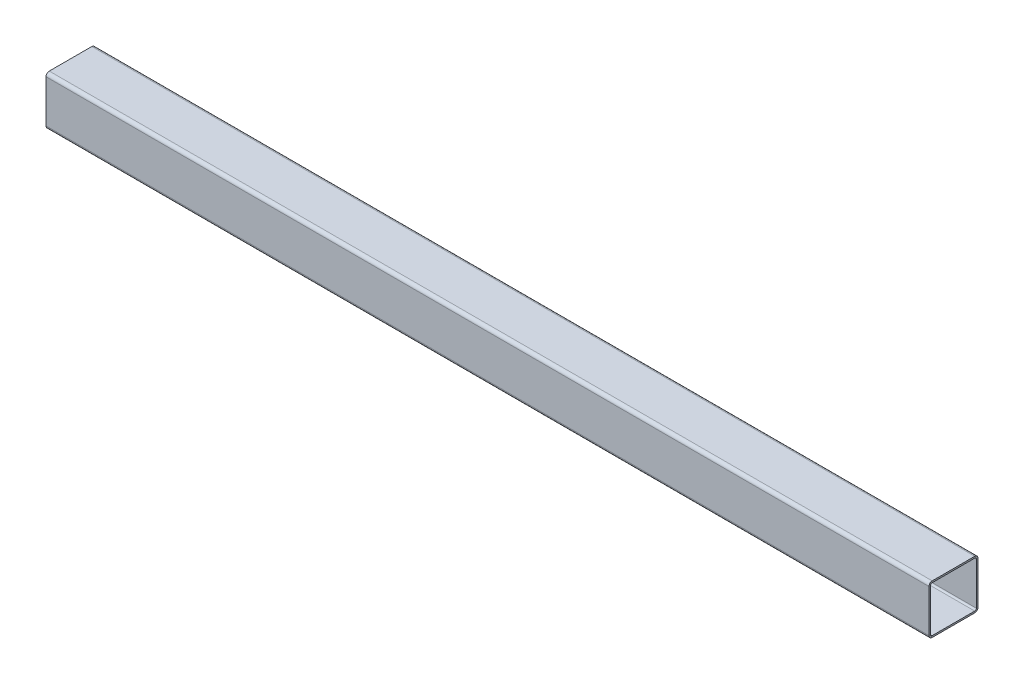
SolidWorks part; units mm, degrees
ref_plane "前视基准面" through (0, 0, 0) normal (0, 0, 1) x (1, 0, 0)
ref_plane "上视基准面" through (0, 0, 0) normal (0, 1, 0) x (1, 0, 0)
ref_plane "右视基准面" through (0, 0, 0) normal (1, 0, 0) x (0, 0, -1)
sketch "草图1" plane through (0, 0, 0) normal (0, 0, 1) x (1, 0, 0)
  line L0 (-1350, 0) -> (1350, 0)
  point P4 (0, 0)
  dimension "D1" = 2700
other "Gb／6728-1986方形空心型钢 150 X 150 X 5(1)"
ref_plane "基准面1" through (-1350, 0, 0) normal (1, 0, 0) x (0, 1, 0)
sketch "Sketch1" plane through (-1350, 0, 0) normal (1, 0, 0) x (0, 1, 0)
  line L0 (-65, -70) -> (65, -70)
  line L1 (-70, -65) -> (-70, 65)
  line L2 (65, 70) -> (-65, 70)
  line L3 (70, 65) -> (70, -65)
  line L4 (-65, -75) -> (65, -75)
  line L5 (-75, -65) -> (-75, 65)
  line L6 (65, 75) -> (-65, 75)
  line L7 (75, 65) -> (75, -65)
  arc A0 (75, 65) -> (65, 75) centre (65, 65) ccw
  arc A1 (65, -75) -> (75, -65) centre (65, -65) ccw
  arc A2 (-75, -65) -> (-65, -75) centre (-65, -65) ccw
  arc A3 (-65, 75) -> (-75, 65) centre (-65, 65) ccw
  arc A4 (-65, 70) -> (-70, 65) centre (-65, 65) ccw
  arc A5 (70, 65) -> (65, 70) centre (65, 65) ccw
  arc A6 (65, -70) -> (70, -65) centre (65, -65) ccw
  arc A7 (-70, -65) -> (-65, -70) centre (-65, -65) ccw
  point P0 (-75, 0)
  point P1 (75, 0)
  point P2 (0, 75)
  point P3 (0, -75)
  point P4 (0, 0)
  point P5 (-75, -75)
  point P6 (75, -75)
  point P7 (75, 75)
  point P8 (-75, 75)
  point P33 (0, 0)
  dimension "D1" = 10
  dimension "Thickness" = 5
  dimension "V_leg" = 150
